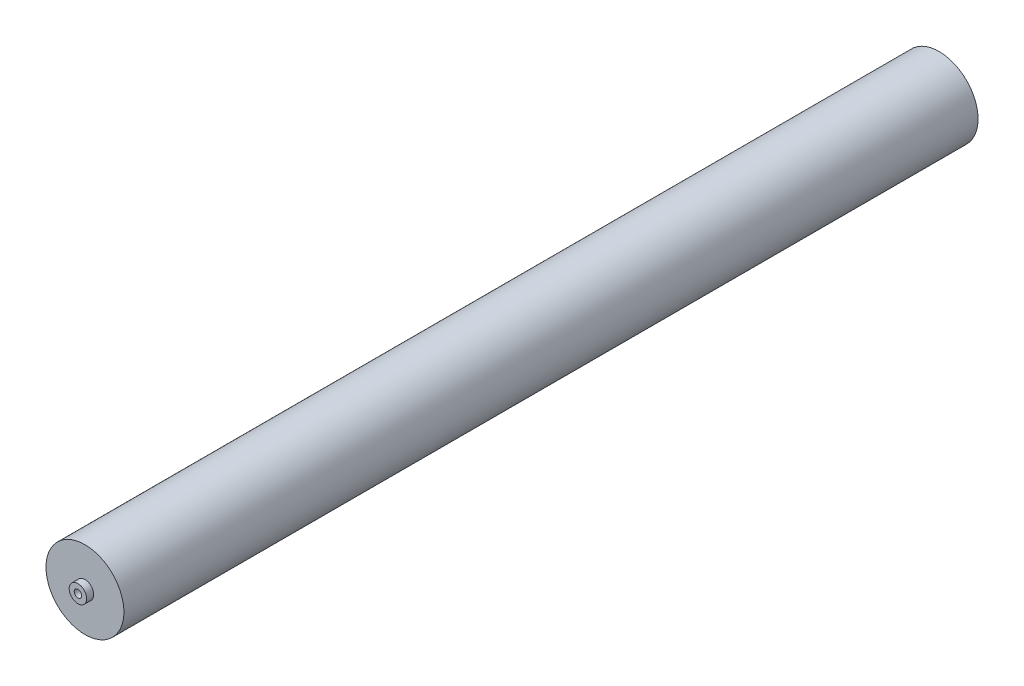
SolidWorks part; units mm, degrees
ref_plane "前视基准面" through (0, 0, 0) normal (0, 0, 1) x (1, 0, 0)
ref_plane "上视基准面" through (0, 0, 0) normal (0, 1, 0) x (1, 0, 0)
ref_plane "右视基准面" through (0, 0, 0) normal (1, 0, 0) x (0, 0, -1)
sketch "草图1" plane through (0, 0, 0) normal (0, 0, 1) x (1, 0, 0)
  circle A0 centre (0, 0) radius 44.5
  dimension "D1" = 89
extrude "凸台-拉伸1" add sketch "草图1" along normal blind 976
sketch "草图2" plane through (0, 0, 976) normal (0, 0, 1) x (1, 0, 0)
  circle A0 centre (0, 0) radius 10
  dimension "D1" = 20
extrude "凸台-拉伸2" add sketch "草图2" along normal blind 8
sketch "草图3" plane through (0, 0, 0) normal (0, 0, -1) x (-1, 0, 0)
  circle A0 centre (0, 0) radius 10
  dimension "D1" = 20
extrude "凸台-拉伸3" add sketch "草图3" along normal blind 8
sketch "草图6" plane through (0, 0, -8) normal (0, 0, -1) x (-1, 0, 0)
  circle A0 centre (0, 0) radius 5
  dimension "D1" = 10
hole_wizard "M10 螺纹孔1" positions "草图7" profile "草图8" tap size "M10" standard "GB"
sketch "草图7" plane through (0, 0, -8) normal (0, 0, -1) x (-1, 0, 0)
  point P0 (0, 0)
cosmetic thread "孔螺蚊线1" parameters "D2"=10
sketch "草图8" plane through (0, 0, -8) normal (1, 0, 0) x (0, 1, 0)
  line L0 (0, 0) -> (0, 25.0537)
  line L1 (0, 25.0537) -> (4.25, 22.5)
  line L2 (4.25, 22.5) -> (4.25, 0)
  line L5 (4.25, 0) -> (0, 0)
  line L10 (0, 25.0537) -> (-4.25, 22.5) construction
  line L11 (0, -6.35) -> (0, 107.95) construction
  dimension "螺纹孔钻头直径" = 8.5
  dimension "螺纹孔钻头深度" = 22.5
  dimension "导头角度" = 118
hole_wizard "M10 螺纹孔2" positions "草图9" profile "草图10" tap size "M10" standard "GB"
sketch "草图9" plane through (0, 0, 984) normal (0, 0, 1) x (1, 0, 0)
  point P0 (0, 0)
sketch "草图10" plane through (0, 0, 984) normal (1, 0, 0) x (0, -1, 0)
  line L0 (0, 0) -> (0, 25.0537)
  line L1 (0, 25.0537) -> (4.25, 22.5)
  line L2 (4.25, 22.5) -> (4.25, 0)
  line L5 (4.25, 0) -> (0, 0)
  line L10 (0, 25.0537) -> (-4.25, 22.5) construction
  line L11 (0, -6.35) -> (0, 107.95) construction
  dimension "螺纹孔钻头直径" = 8.5
  dimension "螺纹孔钻头深度" = 22.5
  dimension "导头角度" = 118
cosmetic thread "孔螺蚊线2"
ref_plane "基准面1" through (0, 0, 488) normal (0, 0, 1) x (1, 0, 0)
sketch "草图11" plane through (0, 0, 488) normal (0, 0, 1) x (1, 0, 0)
  circle A0 centre (0, 0) radius 7.5
  dimension "D1" = 15
extrude "切除-拉伸1" cut sketch "草图11" against normal mid plane 976
